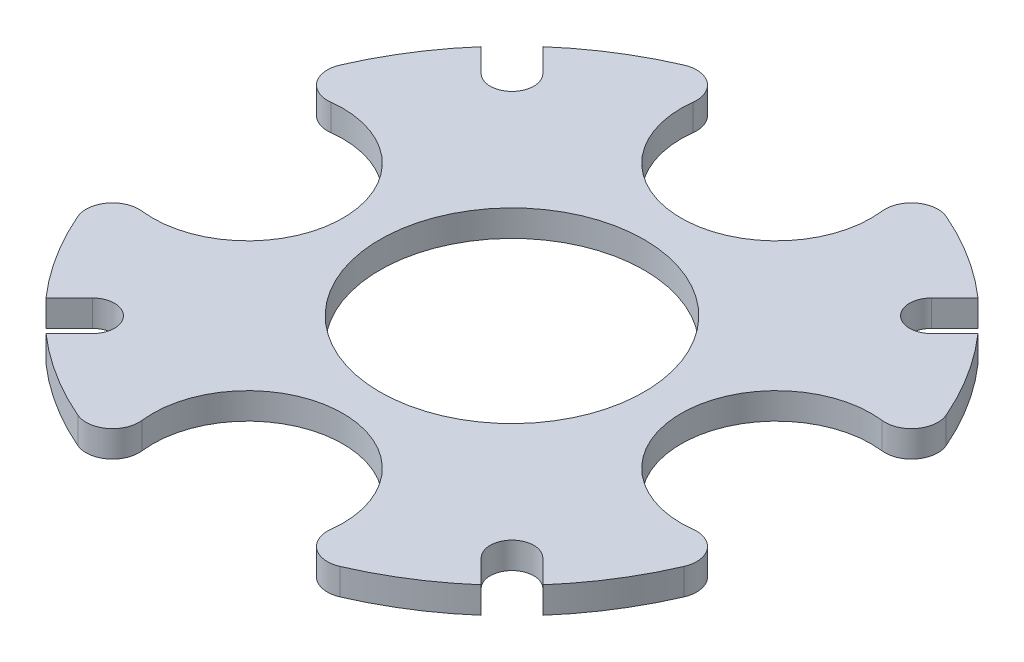
from build123d import *

# Parameters (mm, degrees)
SKETCH4_R           = 5
BOSS_EXTRUDE1_DEPTH = 1


with BuildPart() as part:
    # Sketch4 → Boss-Extrude1 (new body)
    with BuildSketch(Plane(origin=(0, 0, 0), x_dir=(1, 0, 0), z_dir=(0, 1, 0))):
        with BuildLine():
            Line((-7.353910524, -8.520636713), (-8.236199678, -9.402925867))
            ThreePointArc((-8.236199678, -9.402925867), (-6.68048223, -10.565091442), (-4.963540243, -11.472282609))
            ThreePointArc((-4.963540243, -11.472282609), (-3.967940107, -11.355610167), (-3.573748975, -10.433956522))
            ThreePointArc((-3.573748975, -10.433956522), (0, -6.4), (3.573748975, -10.433956522))
            ThreePointArc((3.573748975, -10.433956522), (3.967940107, -11.355610167), (4.963540243, -11.472282609))
            ThreePointArc((4.963540243, -11.472282609), (6.68048223, -10.565091442), (8.236199678, -9.402925867))
            Line((8.236199678, -9.402925867), (7.353910524, -8.520636713))
            ThreePointArc((7.353910524, -8.520636713), (7.353910524, -7.353910524), (8.520636713, -7.353910524))
            Line((8.520636713, -7.353910524), (9.402925867, -8.236199678))
            ThreePointArc((9.402925867, -8.236199678), (10.565091442, -6.68048223), (11.472282609, -4.963540243))
            ThreePointArc((11.472282609, -4.963540243), (11.355610167, -3.967940107), (10.433956522, -3.573748975))
            ThreePointArc((10.433956522, -3.573748975), (6.4, 0), (10.433956522, 3.573748975))
            ThreePointArc((10.433956522, 3.573748975), (11.355610167, 3.967940107), (11.472282609, 4.963540243))
            ThreePointArc((11.472282609, 4.963540243), (10.565091442, 6.68048223), (9.402925867, 8.236199678))
            Line((9.402925867, 8.236199678), (8.520636713, 7.353910524))
            ThreePointArc((8.520636713, 7.353910524), (7.353910524, 7.353910524), (7.353910524, 8.520636713))
            Line((7.353910524, 8.520636713), (8.236199678, 9.402925867))
            ThreePointArc((8.236199678, 9.402925867), (6.68048223, 10.565091442), (4.963540243, 11.472282609))
            ThreePointArc((4.963540243, 11.472282609), (3.967940107, 11.355610167), (3.573748975, 10.433956522))
            ThreePointArc((3.573748975, 10.433956522), (0, 6.4), (-3.573748975, 10.433956522))
            ThreePointArc((-3.573748975, 10.433956522), (-3.967940107, 11.355610167), (-4.963540243, 11.472282609))
            ThreePointArc((-4.963540243, 11.472282609), (-6.68048223, 10.565091442), (-8.236199678, 9.402925867))
            Line((-8.236199678, 9.402925867), (-7.353910524, 8.520636713))
            ThreePointArc((-7.353910524, 8.520636713), (-7.353910524, 7.353910524), (-8.520636713, 7.353910524))
            Line((-8.520636713, 7.353910524), (-9.402925867, 8.236199678))
            ThreePointArc((-9.402925867, 8.236199678), (-10.565091442, 6.68048223), (-11.472282609, 4.963540243))
            ThreePointArc((-11.472282609, 4.963540243), (-11.355610167, 3.967940107), (-10.433956522, 3.573748975))
            ThreePointArc((-10.433956522, 3.573748975), (-6.4, 0), (-10.433956522, -3.573748975))
            ThreePointArc((-10.433956522, -3.573748975), (-11.355610167, -3.967940107), (-11.472282609, -4.963540243))
            ThreePointArc((-11.472282609, -4.963540243), (-10.565091442, -6.68048223), (-9.402925867, -8.236199678))
            Line((-9.402925867, -8.236199678), (-8.520636713, -7.353910524))
            ThreePointArc((-8.520636713, -7.353910524), (-7.353910524, -7.353910524), (-7.353910524, -8.520636713))
        make_face()
        with Locations(Location((0, 0, 0), (0, 0, 90))):
            Circle(SKETCH4_R, mode=Mode.SUBTRACT)
    extrude(amount=BOSS_EXTRUDE1_DEPTH)


solid = part.part
